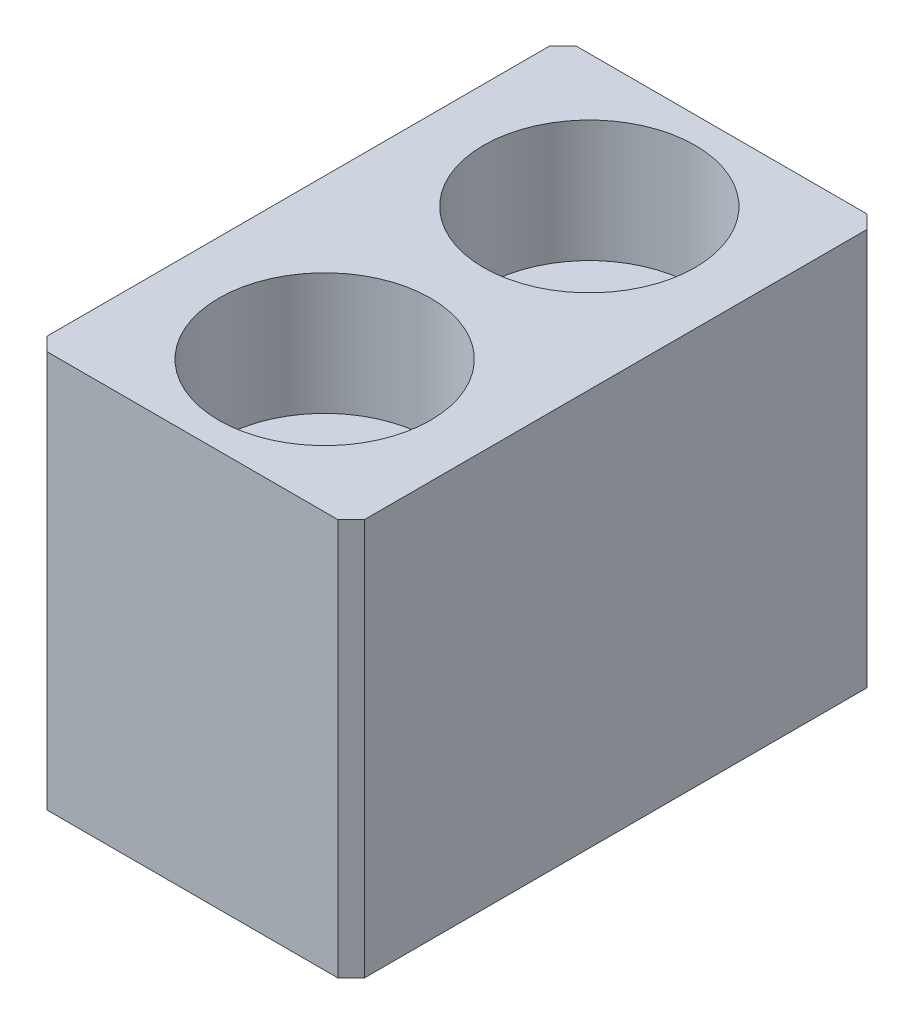
from build123d import *

# Parameters (mm, degrees)
SKETCH_1_W                = 12
SKETCH_1_H                = 20
EXTRUDE_1_DEPTH           = 15
HOLE_WIZARD_1_D           = 4.5
HOLE_WIZARD_1_DEPTH       = 20
HOLE_WIZARD_1_CBORE_D     = 8
HOLE_WIZARD_1_CBORE_DEPTH = 4.6
HOLE_WIZARD_1_TIP         = 1.351936393
CHAMFER_1_SIZE            = 0.5


with BuildPart() as part:
    # 草图1 → 凸台-拉伸1 (new body)
    with BuildSketch(Plane(origin=(0, 0, 0), x_dir=(1, 0, 0), z_dir=(0, 1, 0))):
        Rectangle(SKETCH_1_W, SKETCH_1_H)
    extrude(amount=EXTRUDE_1_DEPTH)

    # 打孔尺寸(%根据)内六角圆柱头螺钉的类型1
    with Locations(Plane(origin=(0, 15, 0), x_dir=(1, 0, 0), z_dir=(0, 1, 0))):
        with Locations((0, 5), (0, -5)):
            CounterBoreHole(HOLE_WIZARD_1_D / 2, HOLE_WIZARD_1_CBORE_D / 2, HOLE_WIZARD_1_CBORE_DEPTH, depth=HOLE_WIZARD_1_DEPTH)
            with Locations((0, 0, -(HOLE_WIZARD_1_DEPTH + HOLE_WIZARD_1_TIP / 2))):  # 118° drill point
                Cone(0, HOLE_WIZARD_1_D / 2, HOLE_WIZARD_1_TIP, mode=Mode.SUBTRACT)

    # 倒角1
    chamfer_1_edges = [part.edges().sort_by_distance(p)[0] for p in [
        (6, 7.5, 10),
        (-6, 7.5, 10),
        (-6, 7.5, -10),
        (6, 7.5, -10),
    ]]
    chamfer(chamfer_1_edges, length=CHAMFER_1_SIZE)


solid = part.part
